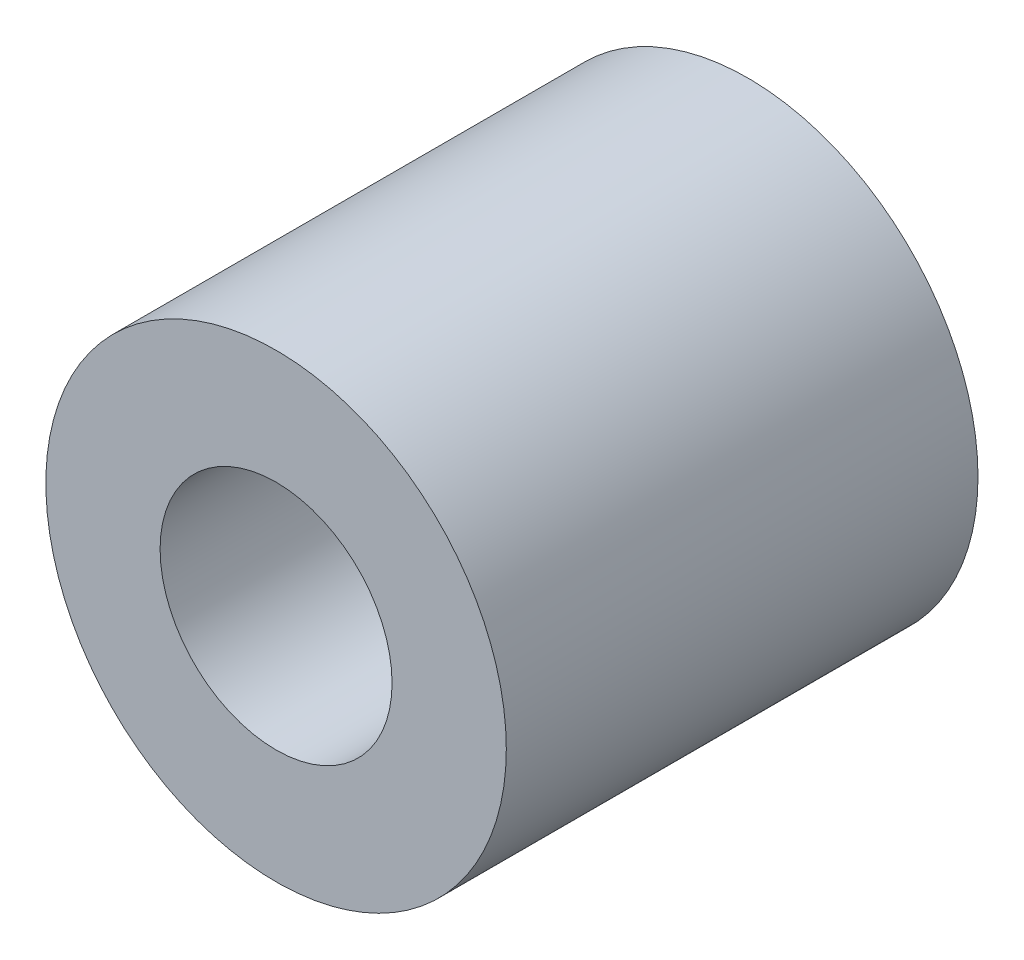
from build123d import *

# Parameters (mm, degrees)
SKETCH1_R           = 5.955
SKETCH1_R_2         = 3
BOSS_EXTRUDE1_DEPTH = 12.2


with BuildPart() as part:
    # Sketch1 → Boss-Extrude1 (new body)
    with BuildSketch(Plane.XY):
        Circle(SKETCH1_R)
        Circle(SKETCH1_R_2, mode=Mode.SUBTRACT)
    extrude(amount=BOSS_EXTRUDE1_DEPTH)


solid = part.part
